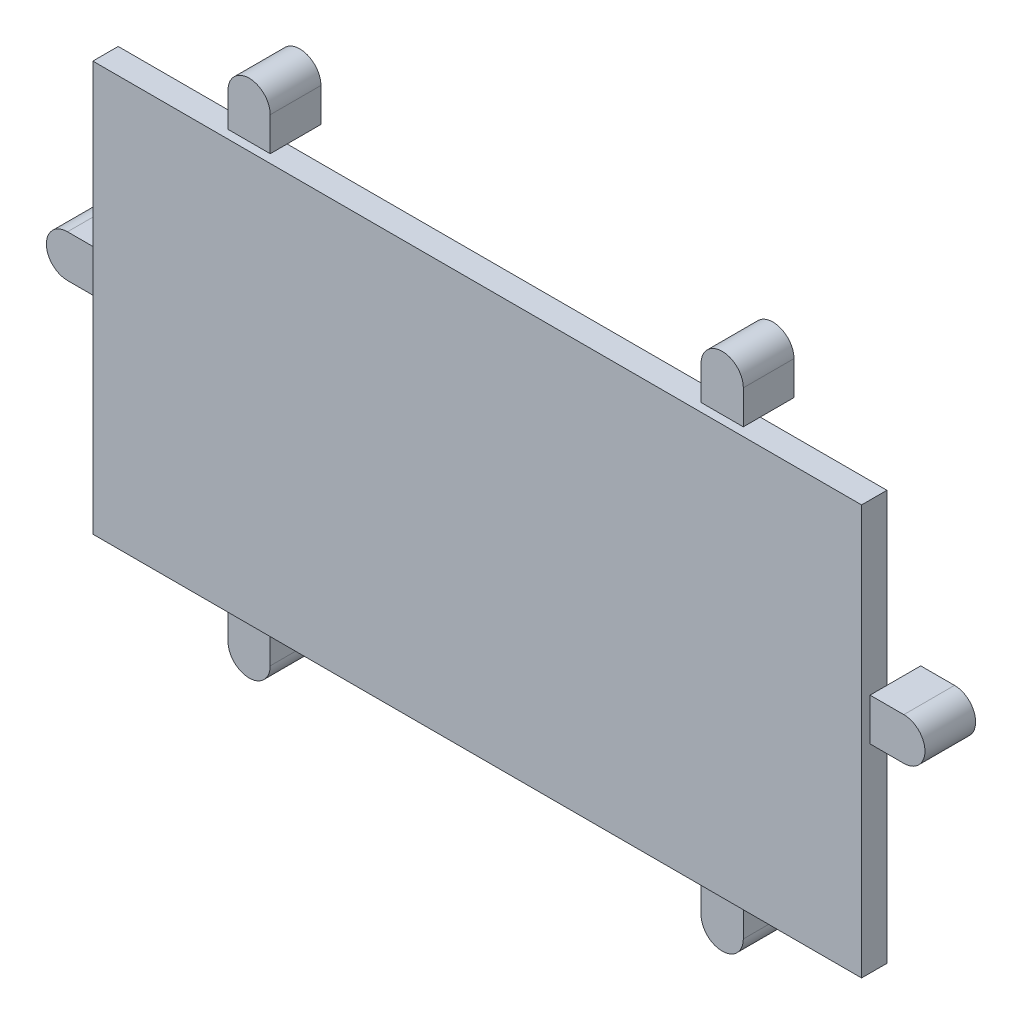
SolidWorks part; units mm, degrees
ref_plane "Front Plane" through (0, 0, 0) normal (0, 0, 1) x (1, 0, 0)
ref_plane "Top Plane" through (0, 0, 0) normal (0, 1, 0) x (1, 0, 0)
ref_plane "Right Plane" through (0, 0, 0) normal (1, 0, 0) x (0, 0, -1)
sketch "Sketch1" plane through (0, 0, 0) normal (0, 0, 1) x (1, 0, 0)
  line L1 (138.0067, -57.9829) -> (-43.9933, -57.9829)
  line L2 (138.0067, -57.9829) -> (138.0067, 39.0171)
  line L3 (138.0067, 39.0171) -> (-43.9933, 39.0171)
  line L4 (-43.9933, -57.9829) -> (-43.9933, 39.0171)
extrude "Boss-Extrude1" add sketch "Sketch1" along normal blind 6
sketch "Sketch2" plane through (0, 0, -8) normal (0, 0, 1) x (1, 0, 0)
  line L6 (108.0067, -65.9829) -> (108.0067, -57.9829)
  line L7 (108.0067, -57.9829) -> (98.0067, -57.9829)
  line L8 (98.0067, -57.9829) -> (98.0067, -65.9829)
  line L9 (108.0067, -65.9829) -> (108.0067, -57.9829)
  line L10 (108.0067, -57.9829) -> (98.0067, -57.9829)
  line L11 (98.0067, -57.9829) -> (98.0067, -65.9829)
  line L15 (138.0067, -0.9829) -> (138.0067, -10.9829)
  line L16 (138.0067, -10.9829) -> (146.0067, -10.9829)
  line L17 (146.0067, -0.9829) -> (138.0067, -0.9829)
  line L18 (138.0067, -0.9829) -> (138.0067, -10.9829)
  line L19 (138.0067, -10.9829) -> (146.0067, -10.9829)
  line L20 (146.0067, -0.9829) -> (138.0067, -0.9829)
  line L24 (108.0067, 39.0171) -> (108.0067, 47.0171)
  line L25 (98.0067, 47.0171) -> (98.0067, 39.0171)
  line L26 (98.0067, 39.0171) -> (108.0067, 39.0171)
  line L27 (108.0067, 39.0171) -> (108.0067, 47.0171)
  line L28 (98.0067, 47.0171) -> (98.0067, 39.0171)
  line L29 (98.0067, 39.0171) -> (108.0067, 39.0171)
  line L33 (-13.9933, 47.0171) -> (-13.9933, 39.0171)
  line L34 (-13.9933, 39.0171) -> (-3.9933, 39.0171)
  line L35 (-3.9933, 39.0171) -> (-3.9933, 47.0171)
  line L36 (-13.9933, 47.0171) -> (-13.9933, 39.0171)
  line L37 (-13.9933, 39.0171) -> (-3.9933, 39.0171)
  line L38 (-3.9933, 39.0171) -> (-3.9933, 47.0171)
  line L42 (-43.9933, -10.9829) -> (-43.9933, -0.9829)
  line L43 (-43.9933, -0.9829) -> (-51.9933, -0.9829)
  line L44 (-51.9933, -10.9829) -> (-43.9933, -10.9829)
  line L45 (-43.9933, -10.9829) -> (-43.9933, -0.9829)
  line L46 (-43.9933, -0.9829) -> (-51.9933, -0.9829)
  line L47 (-51.9933, -10.9829) -> (-43.9933, -10.9829)
  line L51 (-13.9933, -57.9829) -> (-13.9933, -65.9829)
  line L52 (-3.9933, -65.9829) -> (-3.9933, -57.9829)
  line L53 (-3.9933, -57.9829) -> (-13.9933, -57.9829)
  line L54 (-13.9933, -57.9829) -> (-13.9933, -65.9829)
  line L55 (-3.9933, -65.9829) -> (-3.9933, -57.9829)
  line L56 (-3.9933, -57.9829) -> (-13.9933, -57.9829)
  arc A2 (98.0067, -65.9829) -> (108.0067, -65.9829) centre (103.0067, -65.9829) ccw
  arc A3 (98.0067, -65.9829) -> (108.0067, -65.9829) centre (103.0067, -65.9829) ccw
  arc A5 (146.0067, -10.9829) -> (146.0067, -0.9829) centre (146.0067, -5.9829) ccw
  arc A6 (146.0067, -10.9829) -> (146.0067, -0.9829) centre (146.0067, -5.9829) ccw
  arc A8 (108.0067, 47.0171) -> (98.0067, 47.0171) centre (103.0067, 47.0171) ccw
  arc A9 (108.0067, 47.0171) -> (98.0067, 47.0171) centre (103.0067, 47.0171) ccw
  arc A11 (-3.9933, 47.0171) -> (-13.9933, 47.0171) centre (-8.9933, 47.0171) ccw
  arc A12 (-3.9933, 47.0171) -> (-13.9933, 47.0171) centre (-8.9933, 47.0171) ccw
  arc A14 (-51.9933, -0.9829) -> (-51.9933, -10.9829) centre (-51.9933, -5.9829) ccw
  arc A15 (-51.9933, -0.9829) -> (-51.9933, -10.9829) centre (-51.9933, -5.9829) ccw
  arc A17 (-13.9933, -65.9829) -> (-3.9933, -65.9829) centre (-8.9933, -65.9829) ccw
  arc A18 (-13.9933, -65.9829) -> (-3.9933, -65.9829) centre (-8.9933, -65.9829) ccw
  dimension "D1" = 0
  dimension "D2" = 0
  dimension "D3" = 0
  dimension "D4" = 0
  dimension "D5" = 0
  dimension "D6" = 0
extrude "Boss-Extrude2" add sketch "Sketch2" along normal blind 12
